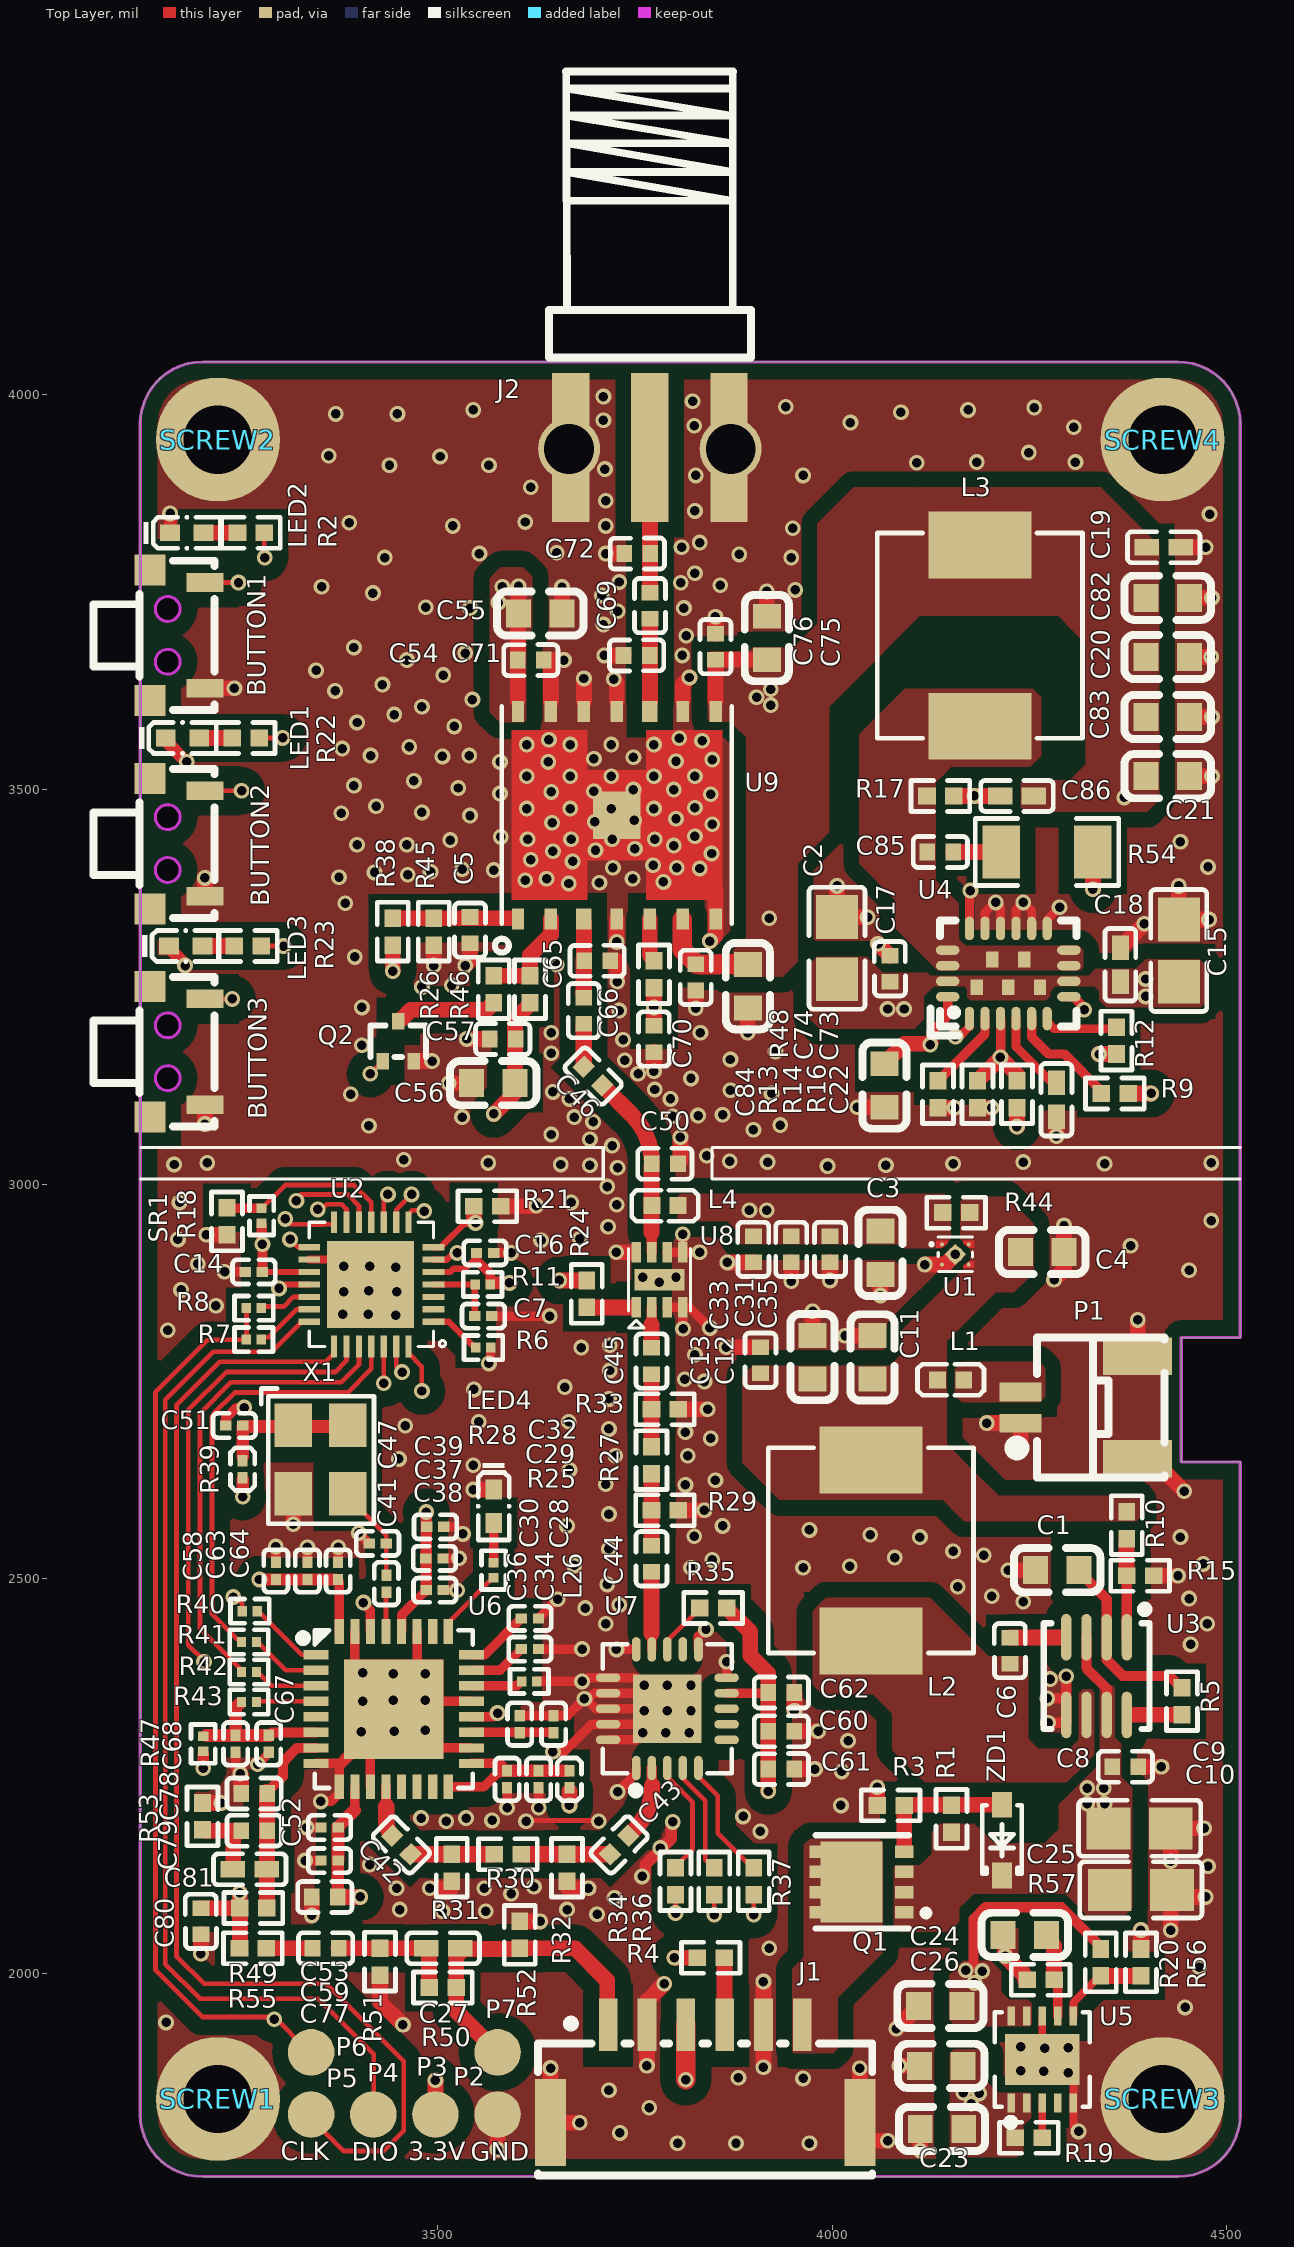
[diagram p0: Top Layer view]
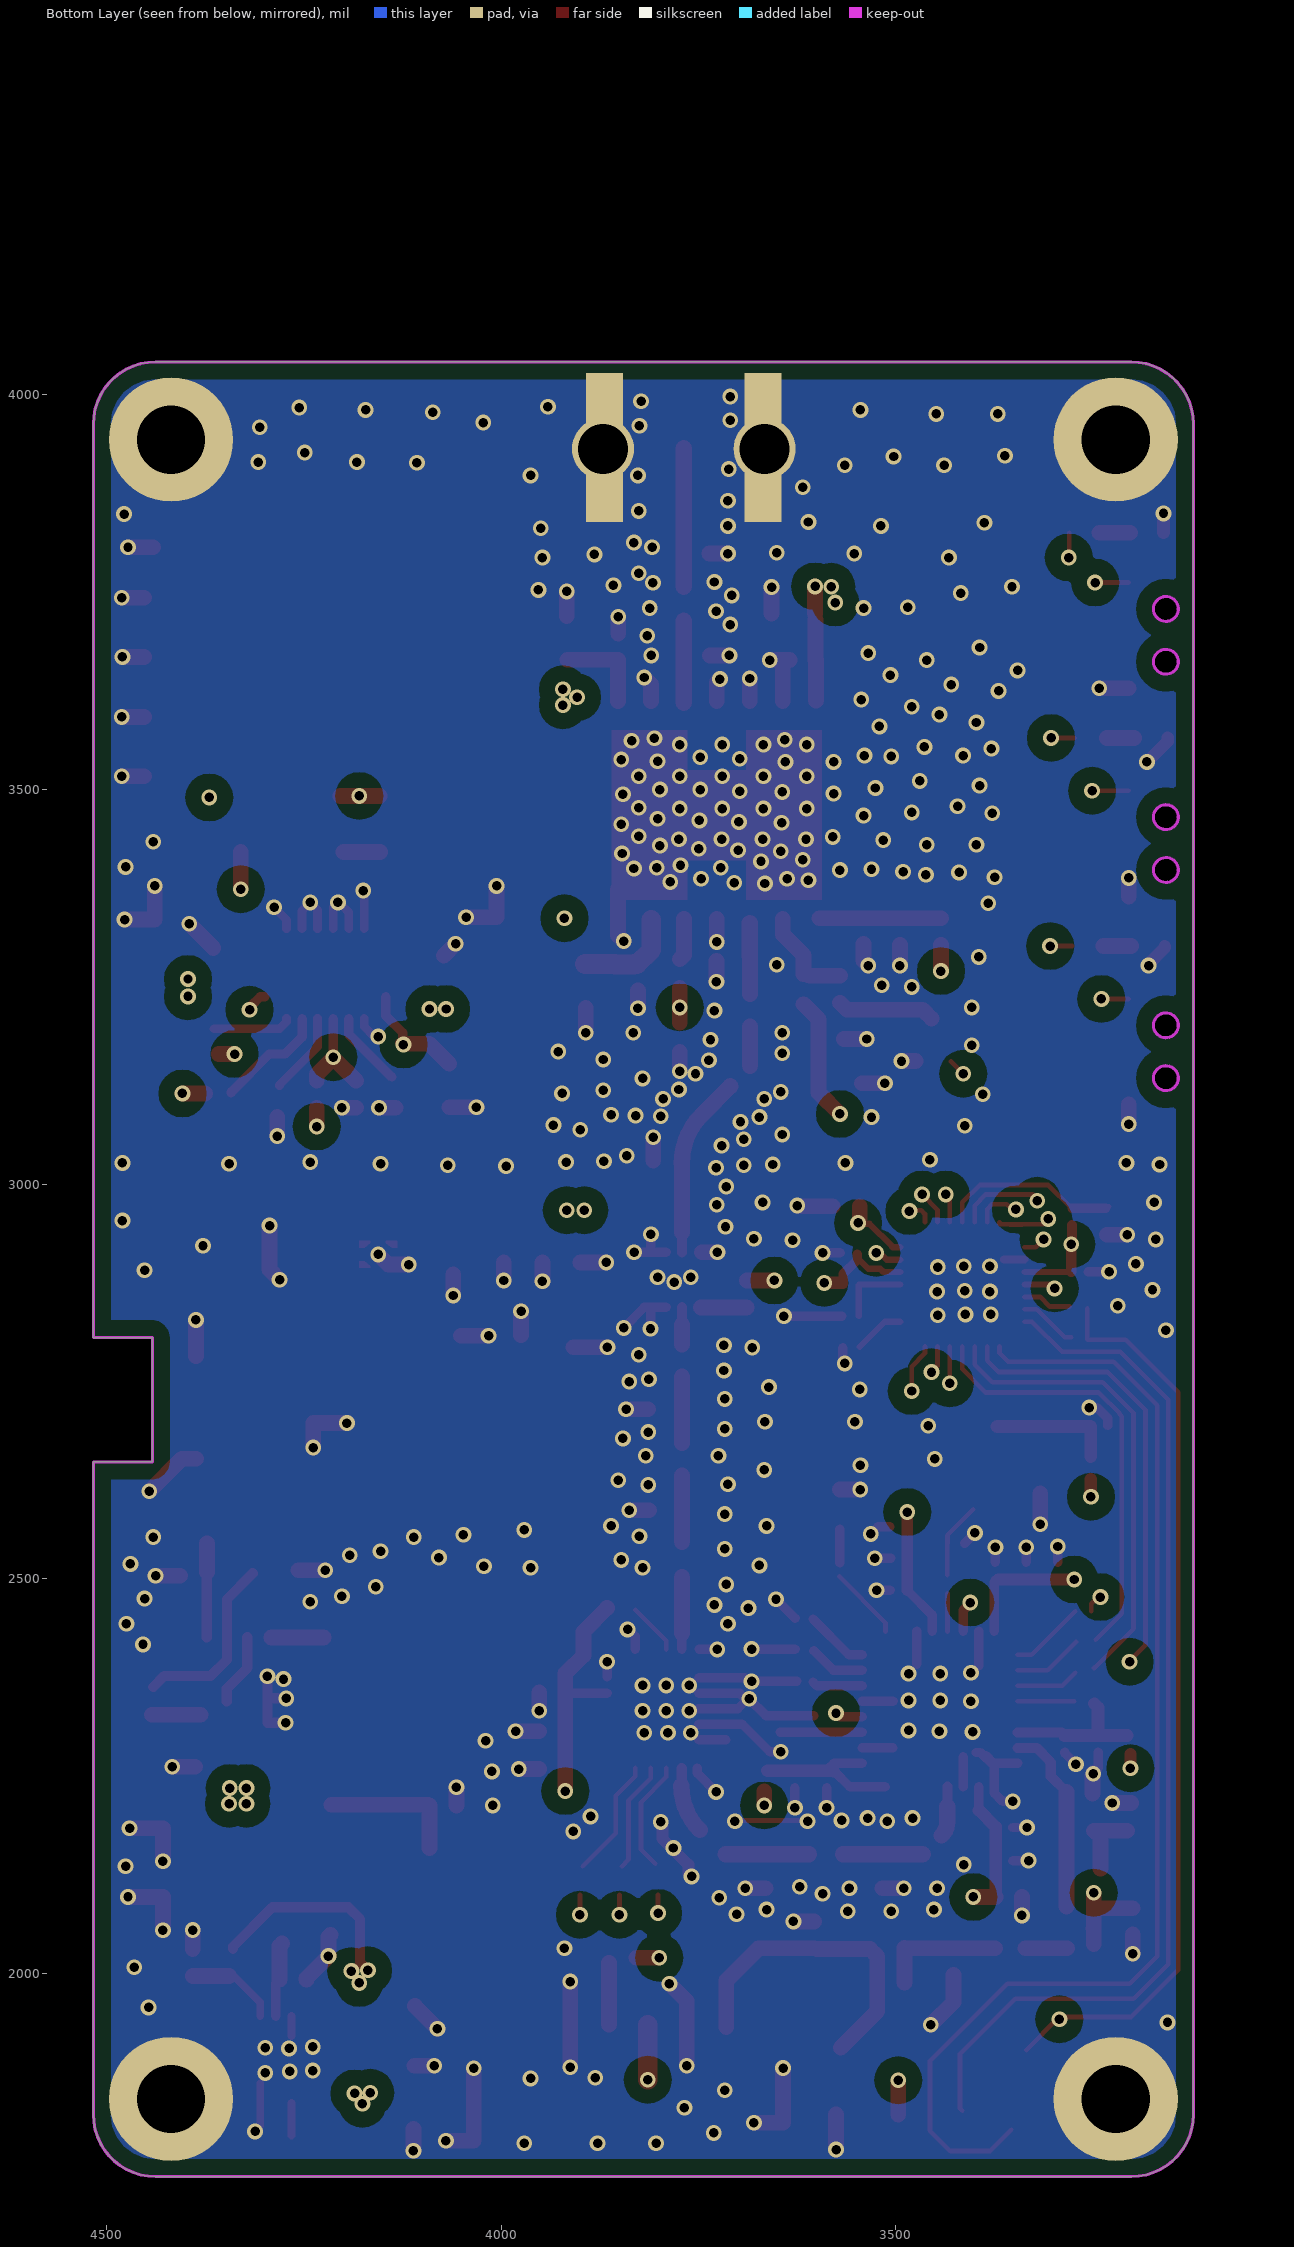
[diagram p1: Bottom Layer view, seen from below]
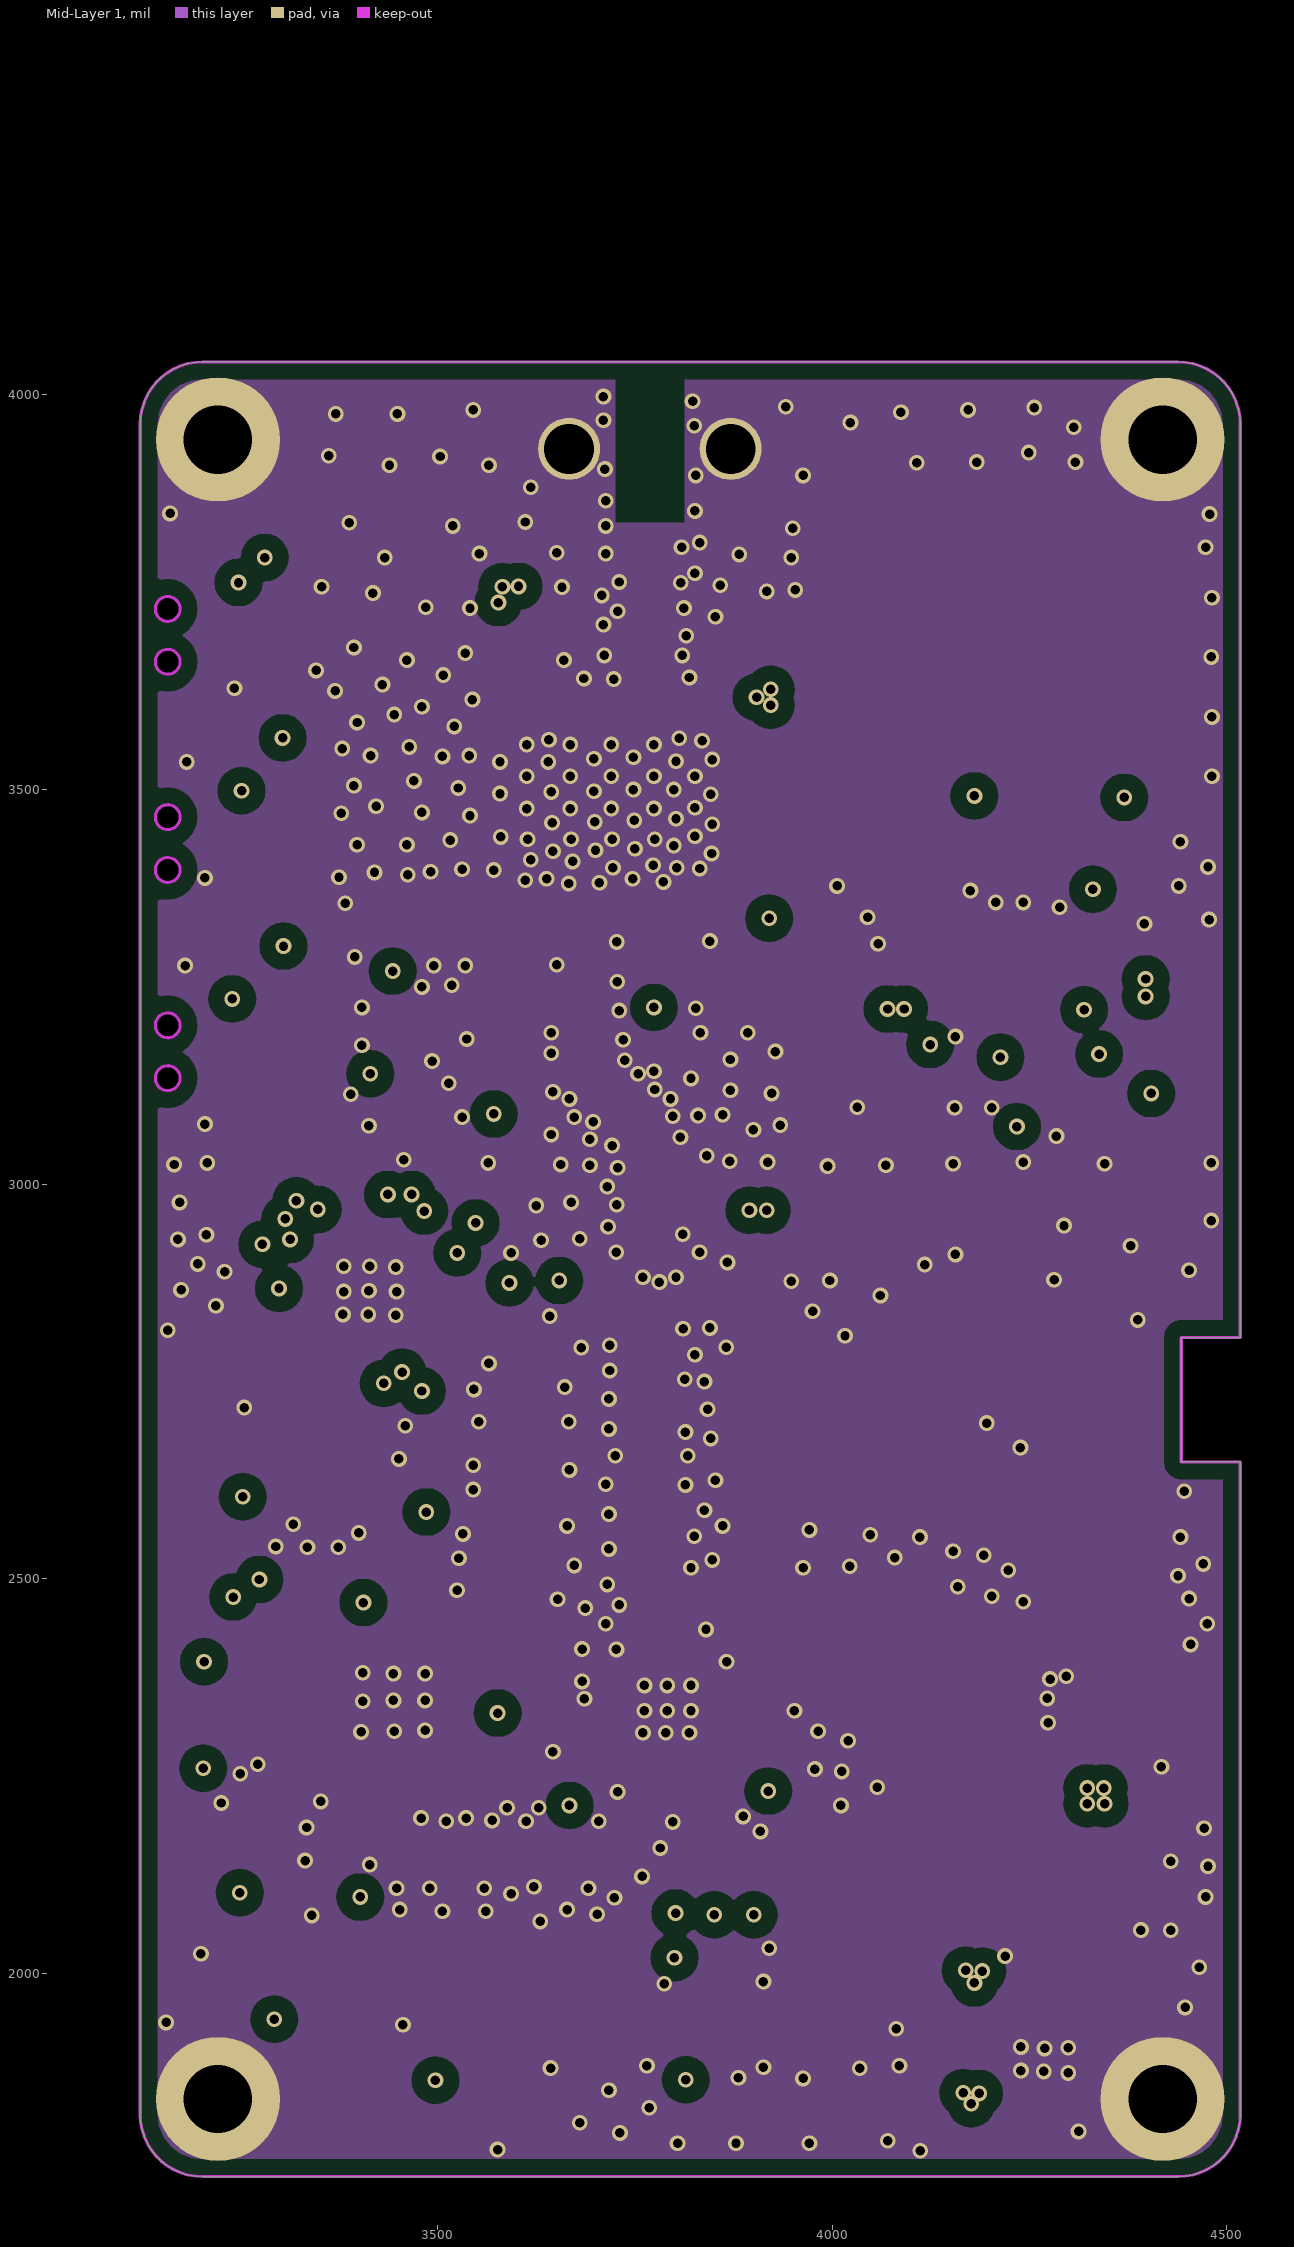
[diagram p2: Mid-Layer 1]
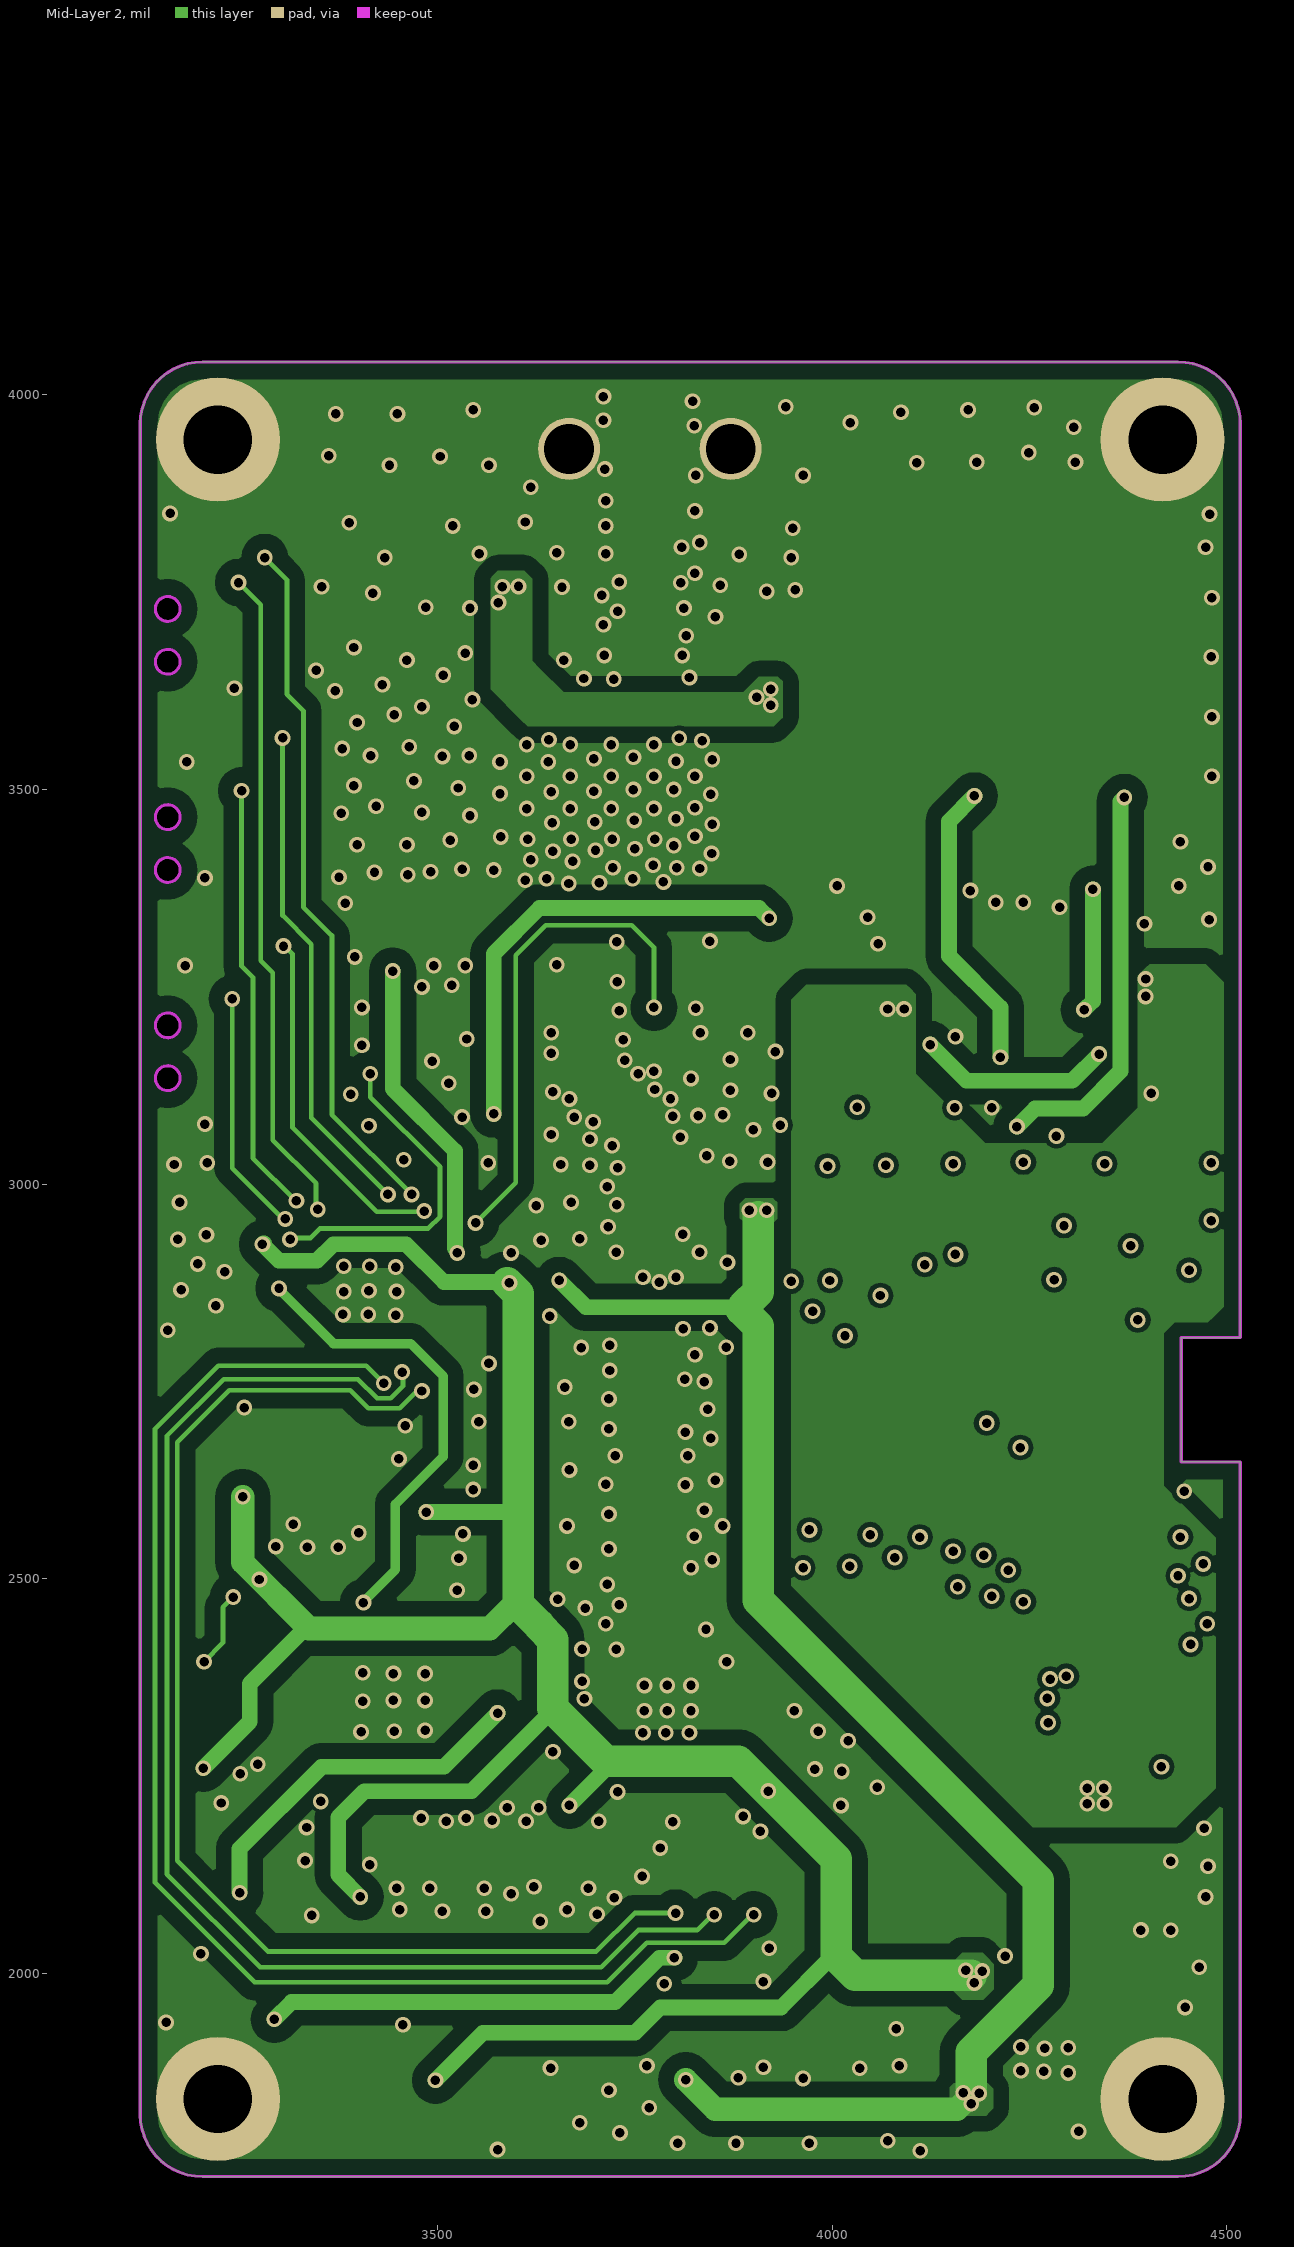
[diagram p3: Mid-Layer 2]
# Altium PCB MISC79034.PcbDoc (part 1 of 2)
Units mil, origin at the board's own origin, x right, y up, seen from the top; angles counter-clockwise.
Board outline 1393.7 x 2299.21 mil, 4 copper layers (Top Layer, Mid-Layer 1, Mid-Layer 2, Bottom Layer); 179 components, 97 nets, 521 pads, 554 vias.

## Layer stack, top to bottom (the 12.6 mil dielectric is the usual default, probably not edited)
Top Layer: signal copper 1.4
Dielectric: core 12.6, FR-4, Dk 4.8
Mid-Layer 1: signal copper 1.4
Dielectric: prepreg 12.6, FR-4, Dk 4.8
Mid-Layer 2: signal copper 1.4
Dielectric: core 12.6, FR-4, Dk 4.8
Bottom Layer: signal copper 1.4

## Board outline
3123.19,1821.38 ccw(c3201.93,1821.38) 3201.93,1742.64 4438.15,1742.64 ccw(c4438.15,1821.38) 4516.89,1821.38 4516.89,2648.15 4442.09,2648.15 4442.09,2805.63 4516.89,2805.63 4516.89,3963.11 ccw(c4438.15,3963.11) 4438.15,4041.85 3201.93,4041.85 ccw(c3201.93,3963.11) 3123.19,3963.11

## Design rules (kind name [scope] priority, off if disabled: settings)
Clearance Clearance_5 [INPOLYGON] p1: gap=6
Clearance [All] p2: gap=6
DiffPairsRouting [All] p1: maxlimit=6 minlimit=6 mostfreqgap=6 maxuncoupledlength=500
HoleSize [All] p1: absolutevalues=TRUE maxlimit=500 minlimit=1 maxpercent=80.000 minpercent=20.000
HoleToHoleClearance [All] p1: gap=0 allowstackedmicrovias=TRUE
MinimumSolderMaskSliver [All] p1: minsoldermaskwidth=0
PlaneClearance [All] p1: clearance=6
PlaneConnect [All] p1: planeconnectstyle=Direct reliefexpansion=20 reliefentries=4 reliefconductorwidth=10 reliefairgap=10
PolygonConnect [All] p1: connectstyle=Direct reliefconductorwidth=10 reliefentries=4 polygonreliefangle="90 Angle"
RoutingVias [All] p1: holewidth=12 width=20 viastyle="Through Hole" minholewidth=12 minwidth=20 maxholewidth=12 maxwidth=20
SilkToSilkClearance [All] p1: silktosilkclearance=0
SilkscreenOverComponentPads [All] p1: minsilkscreentomaskgap=0
SolderMaskExpansion [All] p1: expansion=4
Width [All] p1: maxlimit=100 minlimit=6 preferedwidth=6
20 further rules are at their usual default settings.

## Components (designator, comment, footprint, x,y, rotation, side; value= is the part's Value field where it differs from the comment)
BUTTON1 "TS24CA250GF013" SW-SMD_L4.7-W3.5-P3.35-EH 3170.43,3695.39 r0 top
BUTTON2 "TS24CA250GF013" SW-SMD_L4.7-W3.5-P3.35-EH 3170.43,3431.61 r0 top
BUTTON3 "TS24CA250GF013" SW-SMD_L4.7-W3.5-P3.35-EH 3170.43,3167.83 r0 top
C1 "1uf" C0603 4285,2511 r180 top
C2 "10uF" C0805 4006,3299 r90 top
C3 "1uF" C0603 4061,2913 r270 top
C4 "1uF" C0603 4266,2914 r0 top
C5 "0.1uF" C0402#1 3541,3322 r90 top
C6 "0.1uF" C0402#1 4225,2409 r270 top
C7 "100nf" C0201 3558,2833 r180 top
C8 "100nf" C0402#1 4371.37,2262 r0 top
C9 "10uF" C0805 4389.37,2184 r0 top
C10 "10uF" C0805 4391,2106 r0 top
C11 "22uF" C0603 4051,2780.56 r90 top
C12 "22uF" C0603 3975,2781 r90 top
C13 "100nf" C0402#1 3909,2777 r90 top
C14 "100nf" C0201 3267.2,2889 r180 top
C15 "10uF" C0805 4439,3296 r90 top
C16 "100nf" C0201 3560,2913 r0 top
C17 "100nf" C0402#1 4073,3273 r90 top
C18 "100nf" C0402#2 4365,3278 r90 top
C19 "0.1uF" C0402#2 4420,3807 r180 top
C20 "22uF" C0603 4425,3668 r0 top
C21 "22uF" C0603 4425,3517 r0 top
C22 "33nF" C0402#2 4284,3107 r90 top
C23 "4.7uF" C0603 4139,1803 r0 top
C24 "4.7uF" C0603 4137,1959 r0 top
C25 "4.7uF" C0603 4244,2049 r0 top
C26 "22uF" C0603 4138,1883 r180 top
C27 "150PF" C0402#2 3507,2032 r180 top
C28 "0.1uF" C0201 3647,2316 r270 top
C29 "0.1uF" C0201 3617,2411 r0 top
C30 "1NF" C0201 3604,2316 r90 top
C31 "1UF" C0402#1 3948,2917.46 r90 top
C32 "1NF" C0201 3617,2450 r180 top
C33 "100nf" C0402#1 3900,2917.46 r90 top
C34 "0.1uF" C0201 3628,2246 r90 top
C35 "10PF   50V" C0402#1 3997,2917.46 r270 top
C36 "1NF" C0201 3588,2246 r270 top
C37 "0.1uF" C0201 3496,2526 r180 top
C38 "1NF" C0201 3496.46,2485.62 r0 top
C39 "0.1uF" C0201 3497,2566 r180 top
C41 "1NF" C0201 3435,2494 r90 top
C42 "10PF" C0402#1 3454,2163 r315 top
C43 "10PF" C0402#1 3730,2163 r45 top
C44 "10PF" C0402#1 3771,2525.46 r90 top
C45 "10PF" C0402#1 3771,2776 r90 top
C46 "10PF" C0402#1 3697,3137 r135 top
C47 "1NF" C0201 3424,2545 r180 top
C50 "NC" C0402#1 3788,3026 r0 top
C51 "1NF" C0201 3242.35,2694.31 r0 top
C52 "100PF" C0201 3363,2185 r180 top
C53 "0.1uF" C0201 3363,2143 r0 top
C54 "10PF" C0402#1 3618,3664 r0 top
C55 "4.7UF" C0603 3630,3723 r0 top
C56 "4.7UF" C0603 3570.46,3128 r0 top
C57 "10PF" C0402#1 3582.46,3184 r0 top
C58 "1NF" C0201 3295,2510 r270 top
C59 "10uF" C0402#1 3357,2097 r0 top
C60 "1NF" C0402#1 3935.46,2307 r180 top
C61 "100nf" C0402#1 3935.46,2259 r180 top
C62 "1UF" C0402#1 3935.46,2356 r180 top
C63 "1NF" C0201 3335,2510 r270 top
C64 "1NF" C0201 3374,2510 r90 top
C65 "NC" C0402#1 3702,3283 r0 top
C66 "10PF" C0402#1 3685,3220 r270 top
C67 "1NF" C0201 3286,2291 r270 top
C68 "0.1uF" C0201 3244,2291 r90 top
C69 "10PF" C0402#1 3769,3733 r90 top
C70 "2.2NF" C0402#1 3774,3184 r90 top
C71 "NC" C0402#1 3752,3670 r0 top
C72 "NC" C0402#1 3753,3799 r0 top
C73 "4.7uF" C0603 3893,3251 r270 top
C74 "10PF" C0402#1 3827,3262 r270 top
C75 "4.7UF" C0603 3917,3692 r90 top
C76 "10PF" C0402#1 3852,3681 r90 top
C77 "4.7UF" C0402#1 3358,2032 r180 top
C78 "4.7UF" C0402#1 3267.42,2228 r180 top
C79 "22UF" C0402#1 3267.42,2181 r0 top
C80 "2PF" C0402#1 3200,2066 r90 top
C81 "22uF" C0402#2 3262,2132 r0 top
C82 "22uF" C0603 4425,3743 r0 top
C83 "22uF" C0603 4425,3592 r0 top
C84 "1uf" C0603 4066,3125 r270 top
C85 "0.1uF" C0402#1 4137,3421 r180 top
C86 "390pF" C0402#2 4234,3492 r180 top
J1 "WAFER-GH1. 25-6PWB" SMD_6P-P1.25_XUNPU_WAFER-GH1.25-6PWB 3838.98,1872.99 r0 top locked
J2 "SMA-50KE-3" SMA-FP-945G 3768.86,3931.61 r90 top locked
L1 "MPZ1005S121CT000" L0402 4150,2752 r180 top
L2 "SL0624-100M" IND-SMD_L7.1-W6.6 4049,2536 r90 top
L3 "SL0624-100M" IND-SMD_L7.1-W6.6 4187,3695 r90 top
L4 "33nH" L0402 3788,2973 r0 top
L26 "BLM03PX800SN1D" L0201 3667,2246 r90 top
LED1 "LED" LED0402 3176.8,3565.47 r0 top
LED2 "LED" LED0402 3182.24,3825.31 r0 top
LED3 "LED" LED0402 3180.74,3301.69 r0 top
LED4 "LED" LED0402 3571,2592 r270 top
P1 "WAFER-SHB1.0-2PWB" SMD_2P-WAFER-SHB1.0-2PWB 4312.66,2717.05 r90 top locked
P2 "Pad" PAD 3575.94,1821.38 r0 top locked
P3 "Pad" PAD 3497.2,1821.38 r0 top locked
P4 "Pad" PAD 3418.46,1821.38 r0 top locked
P5 "Pad" PAD 3339.72,1821.38 r0 top locked
P6 "Pad" PAD 3339.72,1900.12 r0 top
P7 "Pad" PAD 3575.94,1900.12 r0 top locked
Q1 "CJAE10P06" DFN-8_L3.0-W3.0-P0.65-BL_G48N03D3 4037,2116 r90 top
Q2 "DULCTU3134K" SOT-523-3_L1.6-W0.8-P0.50-LS1.6-BR-1 3450,3181 r270 top
R1 "50K" R0402 4151,2196 r270 top
R2 "3.3K" R0402 3263.43,3825.31 r180 top
R3 "100K" R0402 4074,2213 r0 top
R4 "1K" R0402 3846,2020 r180 top
R5 "100K" R0402 4443,2345 r270 top
R6 "10K" R0201 3558,2793 r180 top
R7 "22R" R0201 3267,2803 r180 top
R8 "22R" R0201 3267.2,2843 r180 top
R9 "499K" R0402 4358,3115 r0 top
R10 "107K" R0402 4373,2568 r270 top
R11 "10K" R0201 3557,2873 r0 top
R12 "100K" R0402 4360,3182 r270 top
R13 "100K" R0402 4134,3114 r270 top
R14 "10.1K" R0402 4184,3113.96 r270 top
R15 "24.9K" R0402 4390,2504 r0 top
R16 "60K" R0402 4234,3113.96 r90 top
R17 "845K" R0402 4137,3492 r0 top
R18 "10K" R0201 3277,2960 r90 top
R19 "1K" R0402 4249,1792 r180 top
R20 "453K/1%" R0402 4340,2014 r270 top
R21 "10K" R0402 3563,2972 r0 top
R22 "3.3K" R0402 3256.8,3565.47 r180 top
R23 "3.3K" R0402 3259.55,3301.69 r180 top
R24 "3.9K" R0402 3689,2861 r270 top
R25 "4.7K" R0201 3616,2370 r180 top
R26 "1K" R0402 3571,3247 r270 top
R27 "30R" R0402 3771,2650.46 r90 top
R28 "4.7K" R0201 3571,2511 r270 top
R29 "180R" R0402 3788,2587 r0 top
R30 "18R" R0402 3588.92,2151 r0 top
R31 "300R" R0402 3518,2134 r270 top
R32 "300R" R0402 3664,2134 r270 top
R33 "180R" R0402 3788,2715 r0 top
R34 "0R" R0402 3801.37,2116.91 r270 top
R35 "0R" R0402 3849,2463 r0 top
R36 "0R" R0402 3850.37,2116.91 r270 top
R37 "0R" R0402 3900.37,2116.91 r270 top
R38 "0R" R0402 3443,3320 r90 top
R39 "BLM03PX800SN1D" L0201 3253,2639 r90 top
R40 "0R" R0201 3262,2459 r180 top
R41 "0R" R0201 3261,2420 r180 top
R42 "0R" R0201 3261,2382 r180 top
R43 "0R" R0201 3261,2344 r180 top
R44 "NC" R0402 4157,2964 r180 top
R45 "1MR" R0402 3495,3320 r270 top
R46 "0R" R0402 3617,3247 r90 top
R47 "0R" R0201 3203,2291 r270 top
R48 "" R0402 3774,3266 r90 top
R49 "20K" R0402 3266.42,2083 r180 top
R50 "270R" R0402 3506.63,1982.41 r0 top
R51 "10R" R0402 3427,2015 r270 top
R52 "91R" R0402 3604,2049 r90 top
R53 "22R" R0402 3202,2199 r90 top
R54 "4.7R" R1206 4272,3421 r0 top
R55 "2K" R0402 3266,2032 r0 top
R56 "49.9K/1%" R0402 4391,2014 r90 top
R57 "33K" R0402 4264,1992 r0 top
SCREW1 "MARK_4" M2 3221.61,1841.06 r90 top locked
SCREW2 "MARK_4" M2 3221.61,3943.43 r90 top locked
SCREW3 "MARK_4" M2 4418.46,1841.06 r90 top locked
SCREW4 "MARK_4" M2 4418.46,3943.43 r90 top locked
SR1 "SDNT1005X103F3380FTF" R0402 3233,2953 r270 top
U1 "TPS7A2050PDQNR" X2SON-4_L1.0-W1.0-P0.65-TL-EP 4156,2910.99 r0 top
U2 "GD32E230G8U6" QFN-28_L4.0-W4.0-P0.40-BL-EP2.8 3416,2873 r90 top
U3 "AWK6943" QFN-8_L3.0-W3.0-P0.65-BL 4334.8,2376.79 r180 top
U4 "MP4470GL-Z" QFN-20_L4.0-W3.0_MP9447GL 4223,3267 r90 top
U5 "DU3042" WSON-10_L3.0-W3.0-P0.50-BL-EP 4266,1891 r0 top
U6 "GX1288FL" QFN-32_L5.0-W5.0-P0.50 3444.42,2335 r0 top
U7 "ARW621A" QFN-20_L4.0-W4.0-P0.50-TL-EP2.2 3791,2335.46 r90 top
U8 "CBG9092" CBG9092 3781,2879 r90 top
U9 "32A" AU64XX 3727,3467.6 r90 top
X1 "OT322525MJBA4SL" SMD3225 3351.55,2651.31 r270 top
ZD1 "BZT52C15S" SOD-323_L1.7-W1.3-LS2.6-RD 4215,2169 r90 top

## Footprints (in the part's own frame and the unit in brackets; to place one, negate y for a bottom-side part, rotate by r counter-clockwise, add the part's x,y. Pads: shape width x height; smd on the part's side, far side on the other; paste and mask are expansions set on the pad)
AU64XX [mm]
  rect 0.675x0.4 smd paste+0 mask+0.05: 1(-3.337,3.18) 2(-3.337,2.12) 4(-3.337,0) 5(-3.337,-1.06) 6(-3.337,-2.12) 7(-3.337,-3.18) 8(3.338,-3.18) 9(3.338,-2.12) 11(3.338,0) 12(3.338,1.06) 13(3.338,2.12) 14(3.338,3.18)
  rect 0.675x0.5 smd paste+0 mask+0.05: 3(-3.337,1.06) 10(3.338,-1.06)
  rect 1.524x1.524 smd paste+0 mask+0.05: 15(0,0)
  Top Layer region: -2.725,-3.385 -2.725,-0.945 -1.45,-0.945 -1.45,0.945 -2.725,0.945 -2.725,3.385 2.725,3.385 2.725,0.945 1.45,0.945 1.45,-0.945 2.725,-0.945 2.725,-3.385
  silkscreen extent -4.42,-3.7 3.5,3.92
C0201 [mil]
  rect 14.51x12.76 smd paste-3937.01 mask+2: 1(-10.8,0) 2(10.8,0)
  silkscreen extent -27,-15 27,15
C0402#1 [mm]
  rect 0.5x0.54 smd paste+0.051: 1(-0.42,0) 2(0.42,0)
  silkscreen extent -0.87,-0.5 0.87,0.5
C0402#2 [mm]
  rect 0.79x0.54 smd paste-100 mask+0.051: 1(-0.545,0) 2(0.545,0)
  silkscreen extent -1.17,-0.5 1.17,0.5
C0603 [mm]
  rect 0.8x0.9 smd: 1(-0.7,0) 2(0.7,0)
  silkscreen extent -1.39,-0.71 1.39,0.71
C0805 [mm]
  rect 1.41x1.35 smd paste-100 mask+0.051: 1(-1,0) 2(1,0)
  silkscreen extent -1.96,-0.9 1.96,0.9
CBG9092 [mm]
  rect 0.67x0.3 smd: 1(-0.885,0.75) 2(-0.885,0.25) 3(-0.885,-0.25) 4(-0.885,-0.75) 5(0.885,-0.75) 6(0.885,-0.25) 7(0.885,0.25) 8(0.885,0.75)
  rect 0.7x1.6 smd: 9(0,0)
  silkscreen extent -1.55,-1 1,1
DFN-8_L3.0-W3.0-P0.65-BL_G48N03D3 [mm]
  rect 0.4x0.6 smd paste-100 mask+0.051: 1(-0.975,-1.375) 2(-0.325,-1.375) 3(0.325,-1.375) 4(0.975,-1.375) 5(0.975,1.375) 6(0.325,1.375) 7(-0.325,1.375) 8(-0.975,1.375)
  rect 2.6x2 smd paste-100 mask+0.051: 9(0,0.325)
  silkscreen extent -1.5,-2.18 1.5,1.48
IND-SMD_L7.1-W6.6 [mm]
  rect 2.15x3.32 smd: 1(-2.913,0) 2(2.913,0)
  silkscreen extent -3.3,-3.3 3.3,3.3
L0201 [mil]
  rect 14.51x12.76 smd paste-3937.01 mask+2: 1(-10.8,0) 2(10.8,0)
  silkscreen extent -27,-15 27,15
L0402 [mm]
  rect 0.54x0.54 smd paste+0.051: 1(-0.42,0) 2(0.42,0)
  silkscreen extent -1.07,-0.51 1.07,0.49
LED0402 [mm]
  rect 0.636x0.54 smd paste-100 mask+0.051: 1(0.538,0) 2(-0.538,0)
  silkscreen extent -1.39,-0.54 1.09,0.54
M2 [mm]
  round 4 hole 2.2: 1(0,0)
PAD [mm]
  round 1.5 smd: 1(0,0)
QFN-8_L3.0-W3.0-P0.65-BL [mm]
  oval 0.33x1.5 smd: 1(-0.975,-1.25) 2(-0.325,-1.25) 3(0.325,-1.25) 4(0.975,-1.25) 5(0.975,1.25) 6(0.325,1.25) 7(-0.325,1.25) 8(-0.975,1.25)
  silkscreen extent -1.7,-2.27 1.7,1.7
QFN-20_L4.0-W3.0_MP9447GL [mm]
  oval 0.76x0.3 smd paste+0 mask+0.05: 1(-1.45,1.25) 2(-1.45,0.75) 3(-1.45,0.25) 4(-1.45,-0.25) 5(-1.45,-0.75) 6(-1.45,-1.25) 11(1.45,-1.25) 12(1.45,-0.75) 13(1.45,-0.25) 14(1.45,0.25) 15(1.45,0.75) 16(1.45,1.25)
  oval 0.3x0.76 smd paste+0 mask+0.05: 7(-0.75,-1.95) 8(-0.25,-1.95) 9(0.25,-1.95) 10(0.75,-1.95) 17(0.75,1.95) 18(0.25,1.95) 19(-0.25,1.95) 20(-0.75,1.95)
  rect 0.5x0.4 smd: 21(-0.45,1.02) 22(-0.45,0) 23(-0.45,-1.02) 24(0.45,0.51) 25(0.45,-0.51)
  silkscreen extent -2,-2.2 1.7,2.5
QFN-20_L4.0-W4.0-P0.50-TL-EP2.2 [mm]
  oval 0.79x0.28 smd paste-100 mask+0.05: 1(-1.908,1) 2(-1.908,0.5) 3(-1.908,0) 4(-1.908,-0.5) 5(-1.908,-1) 11(1.908,-1) 12(1.908,-0.5) 13(1.908,0) 14(1.908,0.5) 15(1.908,1)
  oval 0.28x0.79 smd paste-100 mask+0.05: 6(-1,-1.908) 7(-0.5,-1.908) 8(0,-1.908) 9(0.5,-1.908) 10(1,-1.908) 16(1,1.908) 17(0.5,1.908) 18(0,1.908) 19(-0.5,1.908) 20(-1,1.908)
  rect 2.2x2.2 smd paste-100 mask+0.05: 21(0,0)
  silkscreen extent -2.76,-2.08 2.08,2.08
QFN-28_L4.0-W4.0-P0.40-BL-EP2.8 [mm]
  rect 0.2x0.7 smd paste-100 mask+0.051: 1(-1.2,-2) 2(-0.8,-2) 3(-0.4,-2) 4(-0.001,-2) 5(0.4,-2) 6(0.8,-2) 7(1.2,-2) 15(1.2,2) 16(0.8,2) 17(0.4,2) 18(0,2) 19(-0.4,2) 20(-0.8,2) 21(-1.2,2)
  rect 0.7x0.2 smd paste-100 mask+0.051: 8(2,-1.2) 9(2,-0.8) 10(2,-0.4) 11(1.999,0) 12(2,0.4) 13(2,0.8) 14(2,1.2) 22(-2,1.2) 23(-2,0.8) 24(-2,0.4) 25(-2,0) 26(-2,-0.4) 27(-2,-0.8) 28(-2,-1.2)
  rect 2.8x2.8 smd paste-100 mask+0.051: 29(0,0.02)
  silkscreen extent -2,-2.39 2,2
QFN-32_L5.0-W5.0-P0.50 [mm]
  rect 0.8x0.3 smd paste-100 mask+0.051: 1(-2.5,1.75) 2(-2.5,1.25) 3(-2.5,0.75) 4(-2.5,0.25) 5(-2.5,-0.25) 6(-2.5,-0.75) 7(-2.5,-1.25) 8(-2.5,-1.75) 17(2.5,-1.75) 18(2.5,-1.25) 19(2.5,-0.75) 20(2.5,-0.25) 21(2.5,0.25) 22(2.5,0.75) 23(2.5,1.25) 24(2.5,1.75)
  rect 0.3x0.8 smd paste-100 mask+0.051: 9(-1.75,-2.5) 10(-1.25,-2.5) 11(-0.75,-2.5) 12(-0.25,-2.5) 13(0.25,-2.5) 14(0.75,-2.5) 15(1.25,-2.5) 16(1.75,-2.5) 25(1.75,2.5) 26(1.25,2.5) 27(0.75,2.5) 28(0.25,2.5) 29(-0.25,2.5) 30(-0.75,2.5) 31(-1.25,2.5) 32(-1.75,2.5)
  rect 3.2x3.2 smd paste-100 mask+0.051: 33(0,0)
  silkscreen extent -3.05,-2.54 2.54,2.54
R0201 [mil]
  rect 11.93x12.76 smd paste-3937.01 mask+2: 1(-9.51,0) 2(9.51,0)
  silkscreen extent -24,-15 24,15
R0402 [mm]
  rect 0.566x0.54 smd paste-100 mask+0.051: 1(-0.433,0) 2(0.433,0)
  silkscreen extent -0.94,-0.5 0.94,0.5
R1206 [mil]
  rect 47.54x66.97 smd paste-3937.01 mask+2: 1(-58.22,0) 2(58.22,0)
  silkscreen extent -91,-42 91,42
SMA-FP-945G [mm] "SMA-FP-945G,侧装,卡板插孔"
  rect 4.8x1.2 smd: 1(0.05,0) 2(0.05,2.55) 2(0.05,-2.55)
  round 2 hole 1.6: 2(0,2.6) 2(0,-2.6)
  rect 4.8x1.2 smd far side: 2(0.05,2.55) 2(0.05,-2.55)
  silkscreen extent 2.94,-3.25 12.15,3.25
SMD3225 [mm]
  rect 1.4x1.2 smd paste+0.051: 1(-1.1,-0.875) 2(1.1,-0.875) 3(1.1,0.875) 4(-1.1,0.875)
  silkscreen extent -2.29,-1.9 2.07,1.72
SMD_2P-WAFER-SHB1.0-2PWB [mm]
  rect 0.6x1.35 smd paste+0 mask+0.05: 1(-0.5,1.887) 2(0.5,1.887)
  rect 1.2x2.22 smd paste+0 mask+0.05: 3(1.65,-1.887) 4(-1.65,-1.887)
  silkscreen extent -2.25,-2.75 2.25,2.2
SMD_6P-P1.25_XUNPU_WAFER-GH1.25-6PWB [mm]
  rect 0.6x1.7 smd paste+0 mask+0.05: 1(-3.125,1.575) 2(-1.875,1.575) 3(-0.625,1.575) 4(0.625,1.575) 5(1.875,1.575) 6(3.125,1.575)
  rect 1x2.8 smd paste+0 mask+0.05: 7(4.975,-1.575) 8(-4.975,-1.575)
  silkscreen extent -5.38,-3.27 5.37,1.74
SOD-323_L1.7-W1.3-LS2.6-RD [mm]
  rect 0.83x0.63 smd paste+0 mask+0.05: 1(1.14,0) 2(-1.14,0)
  silkscreen extent -1.08,-0.64 1.13,0.64
SOT-523-3_L1.6-W0.8-P0.50-LS1.6-BR-1 [mil]
  rect 21x16 smd paste+0 mask+1.97: 1(25.39,-19.68) 2(25.39,19.69)
  rect 21x15.75 smd paste+0 mask+1.97: 3(-25.4,0)
  silkscreen extent -20,-35 20,35
SW-SMD_L4.7-W3.5-P3.35-EH [mm]
  round 0.8 hole 0.8 unplated: 0(-0.315,-0.85) 0(-0.315,0.85)
  rect 1.2x0.6 smd paste+0 mask+0.05: 1(0.882,-1.7) 2(0.882,1.7)
  rect 1x1 smd paste+0 mask+0.05: 3(-0.882,2.1) 4(-0.882,-2.1)
  Keep-Out Layer circle w0.1: c-0.315,-0.85 r0.4
  Keep-Out Layer circle w0.1: c-0.315,0.85 r0.4
  silkscreen extent -2.71,-2.4 1.18,2.4
WSON-10_L3.0-W3.0-P0.50-BL-EP [mm]
  rect 0.25x0.6 smd paste+0.051: 1(-1.001,-1.4) 2(-0.5,-1.4) 3(0,-1.4) 4(0.5,-1.4) 5(1.001,-1.4) 6(1.001,1.4) 7(0.5,1.4) 8(0,1.4) 9(-0.5,1.4) 10(-1.001,1.4)
  rect 2.4x1.65 smd paste+0.051: 11(0,0)
  silkscreen extent -1.52,-2.14 1.52,1.52
X2SON-4_L1.0-W1.0-P0.65-TL-EP [mm]
  round 0.125 smd: 1(-0.43,0.325) 2(-0.43,-0.325) 3(0.43,-0.325) 4(0.43,0.325)
  rect 0.48x0.48 smd rot 45 paste+0 mask+0.05: 5(0,0)
  Top Layer region: 0.61,0.435 0.61,0.215 0.43,0.215 0.25,0.355 0.25,0.435
  Top Layer region: -0.61,0.435 -0.61,0.215 -0.43,0.215 -0.25,0.355 -0.25,0.435
  Top Layer region: -0.61,-0.435 -0.61,-0.215 -0.43,-0.215 -0.25,-0.355 -0.25,-0.435
  Top Layer region: 0.61,-0.435 0.61,-0.215 0.43,-0.215 0.25,-0.355 0.25,-0.435
  silkscreen extent -0.82,-0.55 0.55,0.56

## Part data
BUTTON1 BUTTON2 BUTTON3: library part "TSW 3x6", "3x6 tact switch"
C1 C2 C3 C4 C5 C6 C9 C10 C11 C12 C15 C19 C20 C21 C22 C26 C27 C28 C29 C30 C31 C32 C34 C35 C36 C37 C38 C39 C41 C42 C43 C44 C45 C46 C47 C50 C51 C52 C53 C54 C55 C56 C57 C58 C59 C60 C62 C63 C64 C65 C66 C67 C68 C69 C70 C71 C72 C73 C74 C75 C76 C77 C78 C79 C80 C81 C82 C83 C84 C85 C86: library part 100nf
C23 C24 C25: library part C, "Chip capacitor"
L1 L2 L3 L4: library part L-AL, "Color-ring inductor"
L26 R1 R2 R3 R4 R5 R6 R7 R8 R9 R10 R11 R12 R13 R14 R15 R16 R17 R18 R19 R20 R21 R22 R23 R24 R25 R26 R27 R28 R29 R30 R31 R32 R33 R34 R35 R36 R37 R38 R39 R40 R41 R42 R43 R44 R45 R46 R47 R48 R49 R50 R51 R52 R53 R54 R55 R56 R57: library part R, "Chip resistor"
LED1 LED2 LED3 LED4: library part LED0, "Light-emitting diode"
P1: library part "Header 2", "2P connector"
Q2: library part 2N7002T_C5224243
SCREW1 SCREW2 SCREW3 SCREW4: "MARK Symble"
U3: library part TPS54327DDAR
U5: library part DAC53202RTER, "No Description Available"
U9: library part GCM3527(3.3G-3.8G)
X1: library part XTAL-ACT-4P, "4-pin active crystal oscillator"
ZD1: library part 1N4733, "5.1V/1W Zener diode"

## Via types
v1: diameter 20, hole 12, Top Layer to Bottom Layer, tented both sides, 554 vias

## Nets (pads, with @x,y where several pads share a name; then routed paths per layer and width w, separated by ;. In a path a pad name is that pad's centre, name@x,y a point inside that pad or via, vN(x,y) a via of type N, cw(c..) or ccw(c..) an arc to the next point about the centre after c; other vN are vias at no path point)
3.3V: C14.1 C16.1 C24.2 C37.2 C38.1 C39.2 C52.1 C53.2 C58.2 C59.2 C60.2 C61.2 C62.2 C63.2 C64.1 L26.1 P3.1 R11.2 R18.1 R20.1 R35.2 R39.1 R47.2 U2.5 U2.17 U5.9 U5.10 U6.10 U6.28 U6.32 U7.9 | length 4934.7
  Top Layer w8: C14.1@3283.74,2888.74 U2.17@3337.26,2888.74 ; U2.5@3494.74,2888.75 3515.75,2888.75 3520,2893 3535,2893 C16.1@3549,2907 ; C16.1@3549,2911 C16.1@3549,2913
  Top Layer w12: C64.1@3374,2498 3375.52,2496.48 U6.32@3375.52,2433.42 ; 3394.5,2207.5 3395.21,2208.21 U6.10@3395.21,2236.58 ; U6.28@3454.26,2433.42 3454.26,2454.26 C38.1@3485,2485 ; C16.1@3549,2911 3549,2907 3549,2904.2 3566.51,2886.69 R11.2@3566.51,2873 ; U7.9@3866.1,2355.15 C62.2@3914.85,2355.15
  Top Layer w13: v1@3277,2927 R18.1@3277,2948 ; C14.1@3278,2889 v1(3278,2924) ; v1@4171,2006 4179,2014 4179,2069 4194,2084 4290,2084 4340,2034 R20.1@4340,2031.04
  Top Layer w15: v1(3203,2260) R47.2@3203,2278 ; v1(3274.2,2499.2) C58.2@3295,2499.2 C63.2@3335,2499.2 C64.1@3370.8,2499.2 ; C38.1@3485.66,2485.62 3485.66,2555 ; C39.2@3485.66,2562.66 3485.66,2555 ; v1(3485.66,2584.66) 3485.66,2555
  Top Layer w16: v1(3253,2604) R39.1@3253,2626 ; C59.2@3373.54,2097 C53.2@3373.54,2143 ; C53.2@3373.8,2143 C52.1@3373.8,2185 3373.8,2185.8 3395,2207 ; R11.2@3569,2875 v1@3589,2875
  Top Layer w20: C59.2@3373.54,2097 v1(3402,2097) ; P3.1@3497.2,1821.38 v1(3497.2,1864.8) ; v1(3667,2213) L26.1@3667,2231 ; R35.2@3866.04,2463 3896,2433.04 3896,2403 3918.92,2380.08 C62.2@3918.92,2356 C60.2@3918.92,2307 C61.2@3918.92,2261.92 ; v1(3918.92,2231.08) C61.2@3918.92,2259
  Mid-Layer 2 w20: v1(3203,2260) 3262,2319 3262,2367 3328,2433 ; v1@3279,2925 v1@3280,2925 ; v1@3280,2922 3299,2903 3347,2903 3368,2924 3460,2924 3508,2876 3589,2876 v1@3590,2875 ; v1(3402,2097) 3374,2125 3374,2198 3407,2231 3543,2231 3641,2329 ; v1(3485.66,2584.66) 3586.66,2584.66 ; v1(3497.2,1864.8) 3557.41,1925 3750,1925 3782,1957 3935,1957 3998,2020 ; v1(3667,2213) 3722,2268
  Mid-Layer 2 w30: v1(3253,2604) 3253,2521 3337,2437 3566,2437 3596,2467
  Mid-Layer 2 w40: v1@3588,2875 3602,2861 3602,2468 3628.5,2441.5 ; 3628,2441 3646,2423 3646,2336 3713,2269 3881,2269 v1(3918.92,2231.08) 4005,2145 4005,2022 4029,1998 v1@4176,1998
  other v1: 4180,1988 4190,2003 4169,2004 3591,2875
+5V-FAN: L1.1 P1.2
CPOUT: C78.1 C79.2 C81.2 R49.1 U6.7 | length 240.6
  Top Layer w13: C78.1@3283.96,2229.96 3304,2250 3304,2266.89 3304.88,2267.77 3304.88,2268.88 3321.79,2285.79 U6.7@3346,2285.79
  Top Layer w20: R49.1@3283.96,2085.04 C79.2@3283.96,2181 C78.1@3283.96,2229.96
DSA_CLK: R36.2 U2.27 | length 1745.1
  Top Layer w6: U2.27@3447.5,2794.26 3447.5,2769.5 v1(3455,2762) ; v1(3850.37,2074.37) R36.2@3850.37,2099.87
  Mid-Layer 2 w6: v1@3456,2758 3456,2744 3440.74,2728.74 3423.26,2728.74 3399,2753 3229,2753 3157,2681 3157,2126 3275,2008 3707,2008 3754,2055 3829,2055 v1@3850,2076
DSA_DATA: R34.2 U2.28 | length 1669.8
  Top Layer w6: U2.28@3463.24,2794.26 3463.24,2785.76 3480,2769 v1(3480,2738) ; v1(3801.37,2076.63) R34.2@3801.37,2099.87
  Mid-Layer 2 w6: v1@3477,2741 3452,2716 3412,2716 3389,2739 3236,2739 3170,2673 3170,2143 3285,2028 3701,2028 3749.63,2076.63 v1(3801.37,2076.63)
DSA_LE: R37.2 U2.26 | length 1826.8
  Top Layer w6: v1(3431.74,2747.74) U2.26@3431.74,2794.26 ; v1(3900.37,2074.37) R37.2@3900.37,2099.87
  Mid-Layer 2 w6: v1(3431.74,2747.74) 3409.48,2770 3222,2770 3142,2690 3142,2115 3268,1989 3715,1989 3765,2039 3863,2039 v1@3901,2077